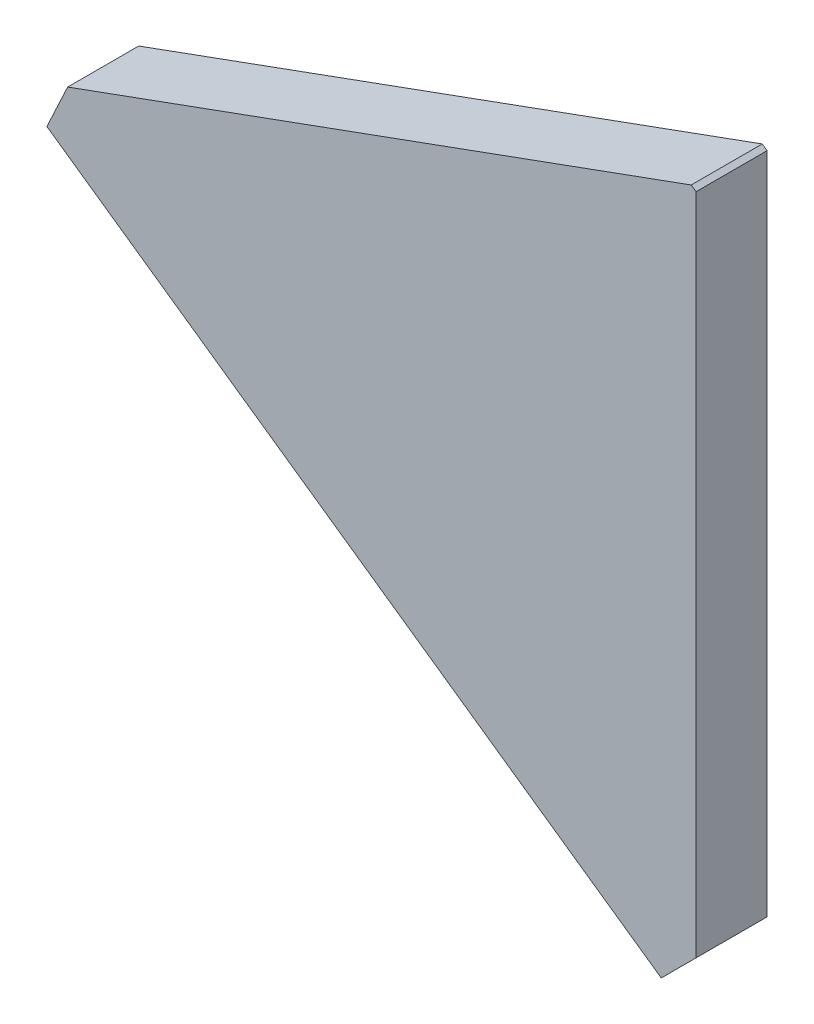
from build123d import *
from OCP.BRepFilletAPI import BRepFilletAPI_MakeChamfer

# Parameters (mm, degrees)
EXTRUDE_START   = -260
EXTRUDE_1_DEPTH = 12
CHAMFER_1_SIZE  = 10
CHAMFER_1_SIZE2 = 7.180150431


with BuildPart() as part:
    # 草图1 → 凸台-拉伸1 (new body)
    with BuildSketch(Plane.XY.offset(EXTRUDE_START)):
        Polygon((-0.819152044, 243.432836403), (-115.534439314, 201.679886421), (0, 120.78180109), (0, 242.859259966), align=None)
    extrude(amount=EXTRUDE_1_DEPTH)

    # 倒角1: one chamfer whose edges measure the first distance from different faces: ONE call of the kernel's chamfer builder (chamfer() names one face for all edges)
    chamfer_1_edges_1 = [part.edges().sort_by_distance(p)[0] for p in [
        (0, 120.78180109, -254),
    ]]
    chamfer_1_side_1 = [part.faces().sort_by_distance(p)[0] for p in [
        (0, 181.820530528, -254),
    ]]
    chamfer_1_edges_2 = [part.edges().sort_by_distance(p)[0] for p in [
        (-115.534439314, 201.679886421, -254),
    ]]
    chamfer_1_side_2 = [part.faces().sort_by_distance(p)[0] for p in [
        (-58.176795679, 222.556361412, -254),
    ]]
    chamfer_1 = BRepFilletAPI_MakeChamfer(part.part.solid().wrapped)
    for e in chamfer_1_edges_1:
        chamfer_1.Add(CHAMFER_1_SIZE, CHAMFER_1_SIZE2, e.wrapped, chamfer_1_side_1[0].wrapped)  # the first distance lies on this face
    for e in chamfer_1_edges_2:
        chamfer_1.Add(CHAMFER_1_SIZE, CHAMFER_1_SIZE2, e.wrapped, chamfer_1_side_2[0].wrapped)  # the first distance lies on this face
    add(Compound.cast(chamfer_1.Shape()), mode=Mode.REPLACE)


solid = part.part
